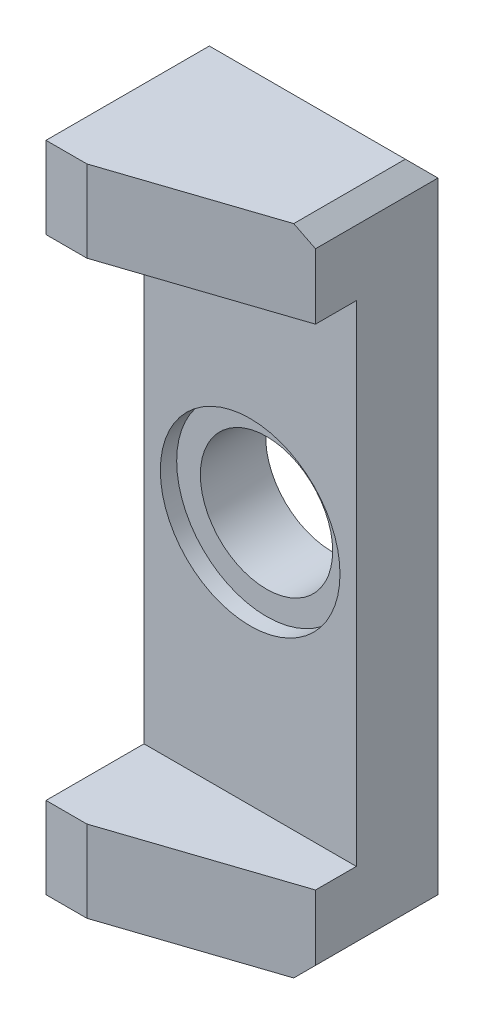
SolidWorks part; units mm, degrees
ref_plane "前视基准面" through (0, 0, 0) normal (0, 0, 1) x (1, 0, 0)
ref_plane "上视基准面" through (0, 0, 0) normal (0, 1, 0) x (1, 0, 0)
ref_plane "右视基准面" through (0, 0, 0) normal (1, 0, 0) x (0, 0, -1)
sketch "草图1" plane through (0, 0, 0) normal (0, 0, 1) x (1, 0, 0)
  line L1 (-13, -40) -> (13, -40)
  line L2 (-13, -40) -> (-13, 40)
  line L3 (-13, 40) -> (13, 40)
  line L4 (13, -40) -> (13, 40)
  line L5 (-13, -40) -> (13, 40) construction
  line L6 (-13, 40) -> (13, -40) construction
  point P0 (0, 0)
  dimension "D1" = 26
  dimension "D2" = 80
extrude "凸台-拉伸1" add sketch "草图1" along normal blind 10 contours L3 L4 L1 L2
sketch "草图2" plane through (0, 0, 10) normal (0, 0, 1) x (1, 0, 0)
  circle A0 centre (0, 0) radius 8.1
  dimension "D1" = 16.2
extrude "切除-拉伸1" cut sketch "草图2" against normal through all
sketch "草图7" plane through (0, 40, 0) normal (0, 1, 0) x (1, 0, 0)
  line L0 (13, -10) -> (13, -15)
  line L2 (-13, -22) -> (-13, -10)
  line L3 (-13, -10) -> (13, -10)
  line L4 (-13, -22) -> (-8, -22)
  line L5 (-8, -22) -> (13, -15)
  dimension "D1" = 5
  dimension "D2" = 12
  dimension "D3" = 5
extrude "凸台-拉伸2" add sketch "草图7" against normal blind 10
mirror "镜向1" about plane through (0, 0, 0) normal (0, 1, 0) of "凸台-拉伸2"
chamfer "倒角1" distance 2 angle 45 2 edges at (13, 40, 7.5) (13, -40, 7.5)
chamfer "倒角2" distance 2 angle 45 2 edges at (-1, -40, 0) (-1, 40, 0)
sketch "草图9" plane through (0, 0, 10) normal (0, 0, -1) x (-1, 0, 0)
  circle A0 centre (0, 0) radius 11
  dimension "D1" = 22
extrude "切除-拉伸2" cut sketch "草图9" along normal blind 2
sketch "草图12" plane through (-13, 0, 0) normal (-1, 0, 0) x (0, 0, 1)
  line L0 (12, 33.4132) -> (12, 46.8033) construction
  line L2 (22, 30) -> (22, 40) construction
  line L3 (0, 0) -> (48.7206, 0) construction
  line L5 (12, -33.4132) -> (12, -46.8033) construction
  point P0 (17, 35)
  point P2 (7, 35)
  point P11 (22, 35)
  point P20 (7, -35)
  point P21 (17, -35)
  dimension "D1" = 10
  dimension "D2" = 10
hole_wizard "M4 螺纹孔1" positions "草图12" profile "草图11" tap size "M4" standard "GB"
sketch "草图11" plane through (-13, 35, 17) normal (0, 1, 0) x (0, 0, 1)
  line L0 (0, 0) -> (0, 11.0914)
  line L1 (0, 11.0914) -> (1.65, 10.1)
  line L2 (1.65, 10.1) -> (1.65, 0)
  line L5 (1.65, 0) -> (0, 0)
  line L10 (0, 11.0914) -> (-1.65, 10.1) construction
  line L11 (0, -6.35) -> (0, 107.95) construction
  dimension "螺纹孔钻头直径" = 3.3
  dimension "螺纹孔钻头深度" = 10.1
  dimension "导头角度" = 118
cosmetic thread "孔螺纹线1" parameters "D1"=8, "D2"=4
cosmetic thread "孔螺纹线2" parameters "D1"=8, "D2"=4
cosmetic thread "孔螺纹线3" parameters "D1"=8, "D2"=4
cosmetic thread "孔螺纹线4" parameters "D1"=8, "D2"=4
